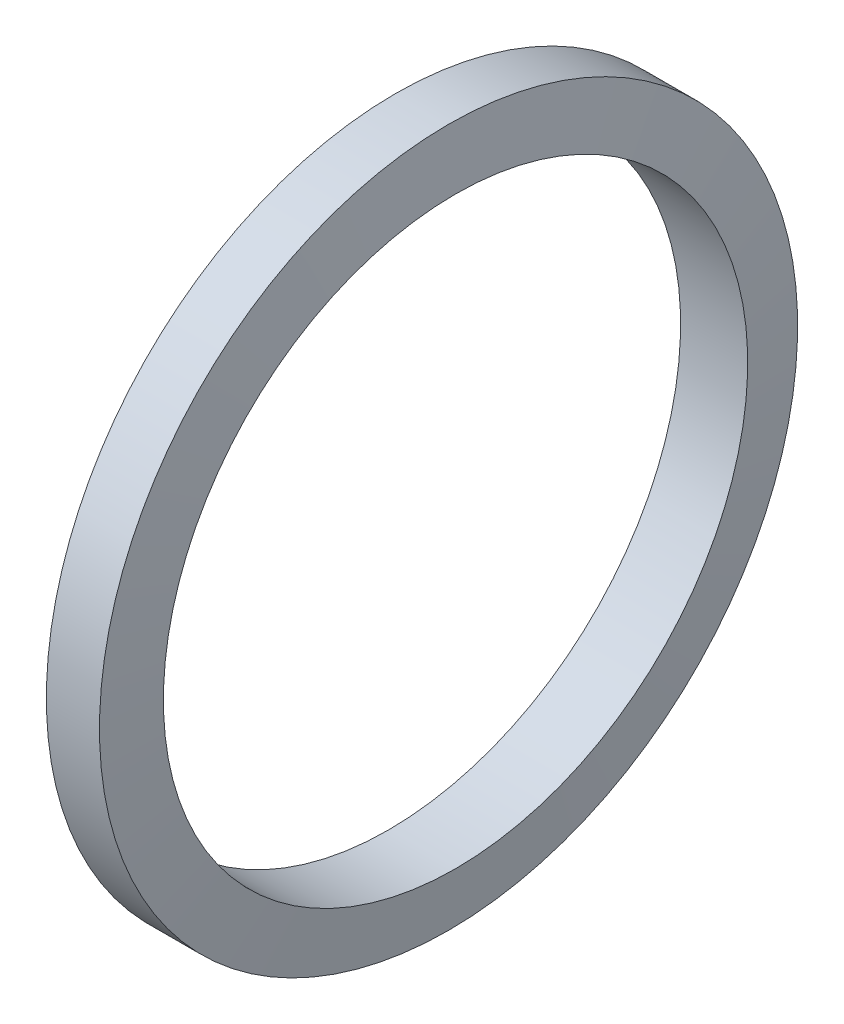
SolidWorks part; units mm, degrees
ref_plane "Front Plane" through (0, 0, 0) normal (0, 0, 1) x (1, 0, 0)
ref_plane "Top Plane" through (0, 0, 0) normal (0, 1, 0) x (1, 0, 0)
ref_plane "Right Plane" through (0, 0, 0) normal (1, 0, 0) x (0, 0, -1)
sketch "Sketch2" plane through (0, 0, 0) normal (0, 0, 1) x (1, 0, 0)
  line L0 (-3.5, 0) -> (3.5, 0)
  line L1 (-3.5, 0) -> (-4.4209, -7.5)
  line L2 (-4.4209, -7.5) -> (4.4209, -7.5)
  line L3 (4.4209, -7.5) -> (3.5, 0)
  line L4 (0, 0) -> (0, 6.27) construction
  line L5 (0, 0) -> (0, -46) construction
  point P4 (0, 0)
  dimension "D1" = 7
  dimension "D2" = 14
  dimension "D3" = 38.5
  dimension "D4" = 46
sketch "Sketch3" plane through (0, 0, 0) normal (1, 0, 0) x (0, 0, -1)
  line L0 (0, 0) -> (0, -46) construction
  circle A0 centre (0, -46) radius 46
sweep "Sweep1" add profiles "Sketch2" path "Sketch3"
